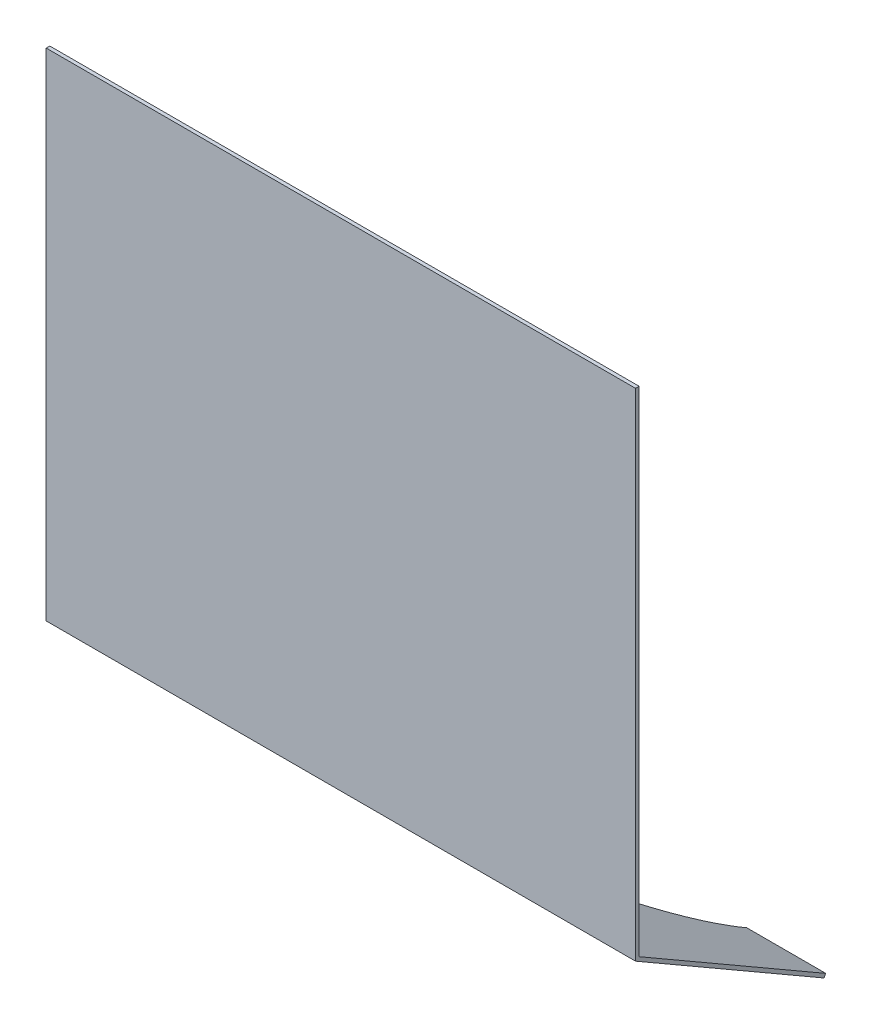
SolidWorks part; units mm, degrees
ref_plane "前视基准面" through (0, 0, 0) normal (0, 0, 1) x (1, 0, 0)
ref_plane "上视基准面" through (0, 0, 0) normal (0, 1, 0) x (1, 0, 0)
ref_plane "右视基准面" through (0, 0, 0) normal (1, 0, 0) x (0, 0, -1)
sketch "草图1" plane through (0, 0, 0) normal (0, 0, 1) x (1, 0, 0)
  line L11 (-164, 137.5) -> (164, 137.5)
  line L12 (-164, 137.5) -> (-164, -137.5)
  line L13 (-164, -137.5) -> (164, -137.5)
  line L14 (164, 137.5) -> (164, -137.5)
  line L15 (-164, 137.5) -> (164, -137.5) construction
  line L16 (-164, -137.5) -> (164, 137.5) construction
  point P0 (0, 0)
  dimension "D1" = 328
  dimension "D2" = 275
extrude "凸台-拉伸1" add sketch "草图1" along normal blind 2
sketch "草图2" plane through (-164, 0, 0) normal (-1, 0, 0) x (0, 0, 1)
  line L0 (0, -137.5) -> (-103.923, -197.5)
  line L1 (0, 137.5) -> (0, -137.5) construction
  line L2 (1, -139.2321) -> (-102.923, -199.2321)
  line L3 (-103.923, -197.5) -> (-102.923, -199.2321)
  line L4 (1, -139.2321) -> (2, -138.6547)
  line L5 (2, -138.6547) -> (2, -137.5)
  line L6 (0, -137.5) -> (2, -137.5)
  dimension "D1" = 60
  dimension "D2" = 120
  dimension "D3" = 2
extrude "凸台-拉伸2" add sketch "草图2" against normal up to surface (328 mm away) up to face at (164, 0, 1)
sketch "草图3" plane through (0, 0, 0) normal (0, 0, 1) x (1, 0, 0)
  line L0 (0, 100.7679) -> (0, -184.2321) construction
  line L1 (7, 100.7679) -> (7, -184.2321)
  line L2 (-7, 100.7679) -> (-7, -184.2321)
  line L3 (30, 100.7679) -> (30, -184.2321) construction
  line L6 (37, 100.7679) -> (37, -184.2321)
  line L9 (23, 100.7679) -> (23, -184.2321)
  line L12 (60, 100.7679) -> (60, -184.2321) construction
  line L15 (67, 100.7679) -> (67, -184.2321)
  line L18 (53, 100.7679) -> (53, -184.2321)
  line L21 (90, 100.7679) -> (90, -184.2321) construction
  line L24 (97, 100.7679) -> (97, -184.2321)
  line L27 (83, 100.7679) -> (83, -184.2321)
  line L30 (120, 100.7679) -> (120, -184.2321) construction
  line L33 (127, 100.7679) -> (127, -184.2321)
  line L36 (113, 100.7679) -> (113, -184.2321)
  line L39 (164, -199.2321) -> (-164, -199.2321) construction
  line L40 (-30, 100.7679) -> (-30, -184.2321) construction
  line L41 (-23, 100.7679) -> (-23, -184.2321)
  line L42 (-37, 100.7679) -> (-37, -184.2321)
  line L43 (-60, 100.7679) -> (-60, -184.2321) construction
  line L44 (-53, 100.7679) -> (-53, -184.2321)
  line L45 (-67, 100.7679) -> (-67, -184.2321)
  line L46 (-90, 100.7679) -> (-90, -184.2321) construction
  line L47 (-83, 100.7679) -> (-83, -184.2321)
  line L48 (-97, 100.7679) -> (-97, -184.2321)
  line L49 (-120, 100.7679) -> (-120, -184.2321) construction
  line L50 (-113, 100.7679) -> (-113, -184.2321)
  line L51 (-127, 100.7679) -> (-127, -184.2321)
  arc A0 (7, 100.7679) -> (-7, 100.7679) centre (0, 100.7679) ccw
  arc A1 (-7, -184.2321) -> (7, -184.2321) centre (0, -184.2321) ccw
  arc A2 (37, 100.7679) -> (23, 100.7679) centre (30, 100.7679) ccw
  arc A3 (23, -184.2321) -> (37, -184.2321) centre (30, -184.2321) ccw
  arc A4 (67, 100.7679) -> (53, 100.7679) centre (60, 100.7679) ccw
  arc A5 (53, -184.2321) -> (67, -184.2321) centre (60, -184.2321) ccw
  arc A6 (97, 100.7679) -> (83, 100.7679) centre (90, 100.7679) ccw
  arc A7 (83, -184.2321) -> (97, -184.2321) centre (90, -184.2321) ccw
  arc A8 (127, 100.7679) -> (113, 100.7679) centre (120, 100.7679) ccw
  arc A9 (113, -184.2321) -> (127, -184.2321) centre (120, -184.2321) ccw
  arc A10 (-23, 100.7679) -> (-37, 100.7679) centre (-30, 100.7679) ccw
  arc A11 (-37, -184.2321) -> (-23, -184.2321) centre (-30, -184.2321) ccw
  arc A12 (-53, 100.7679) -> (-67, 100.7679) centre (-60, 100.7679) ccw
  arc A13 (-67, -184.2321) -> (-53, -184.2321) centre (-60, -184.2321) ccw
  arc A14 (-83, 100.7679) -> (-97, 100.7679) centre (-90, 100.7679) ccw
  arc A15 (-97, -184.2321) -> (-83, -184.2321) centre (-90, -184.2321) ccw
  arc A16 (-113, 100.7679) -> (-127, 100.7679) centre (-120, 100.7679) ccw
  arc A17 (-127, -184.2321) -> (-113, -184.2321) centre (-120, -184.2321) ccw
  point P2 (0, -41.7321)
  point P11 (30, -41.7321)
  point P18 (60, -41.7321)
  point P25 (90, -41.7321)
  point P32 (120, -41.7321)
  point P40 (-30, -41.7321)
  point P47 (-60, -41.7321)
  point P55 (-90, -41.7321)
  point P62 (-120, -41.7321)
  dimension "D2" = 7
  dimension "D6" = 15
sketch "草图4" plane through (0, -103.125, 59.5392) normal (0, 0.866, -0.5) x (1, 0, 0)
  line L0 (164, 188.75) -> (-164, 188.75) construction
  ellipse E0 centre (0, 188.75) end of major axis (120, 188.75) minor radius 100
  point P1 (0, 0)
  dimension "D1" = 188.75
  dimension "D2" = 200
  dimension "D3" = 240
extrude "切除-拉伸1" cut sketch "草图4" against normal blind 10
